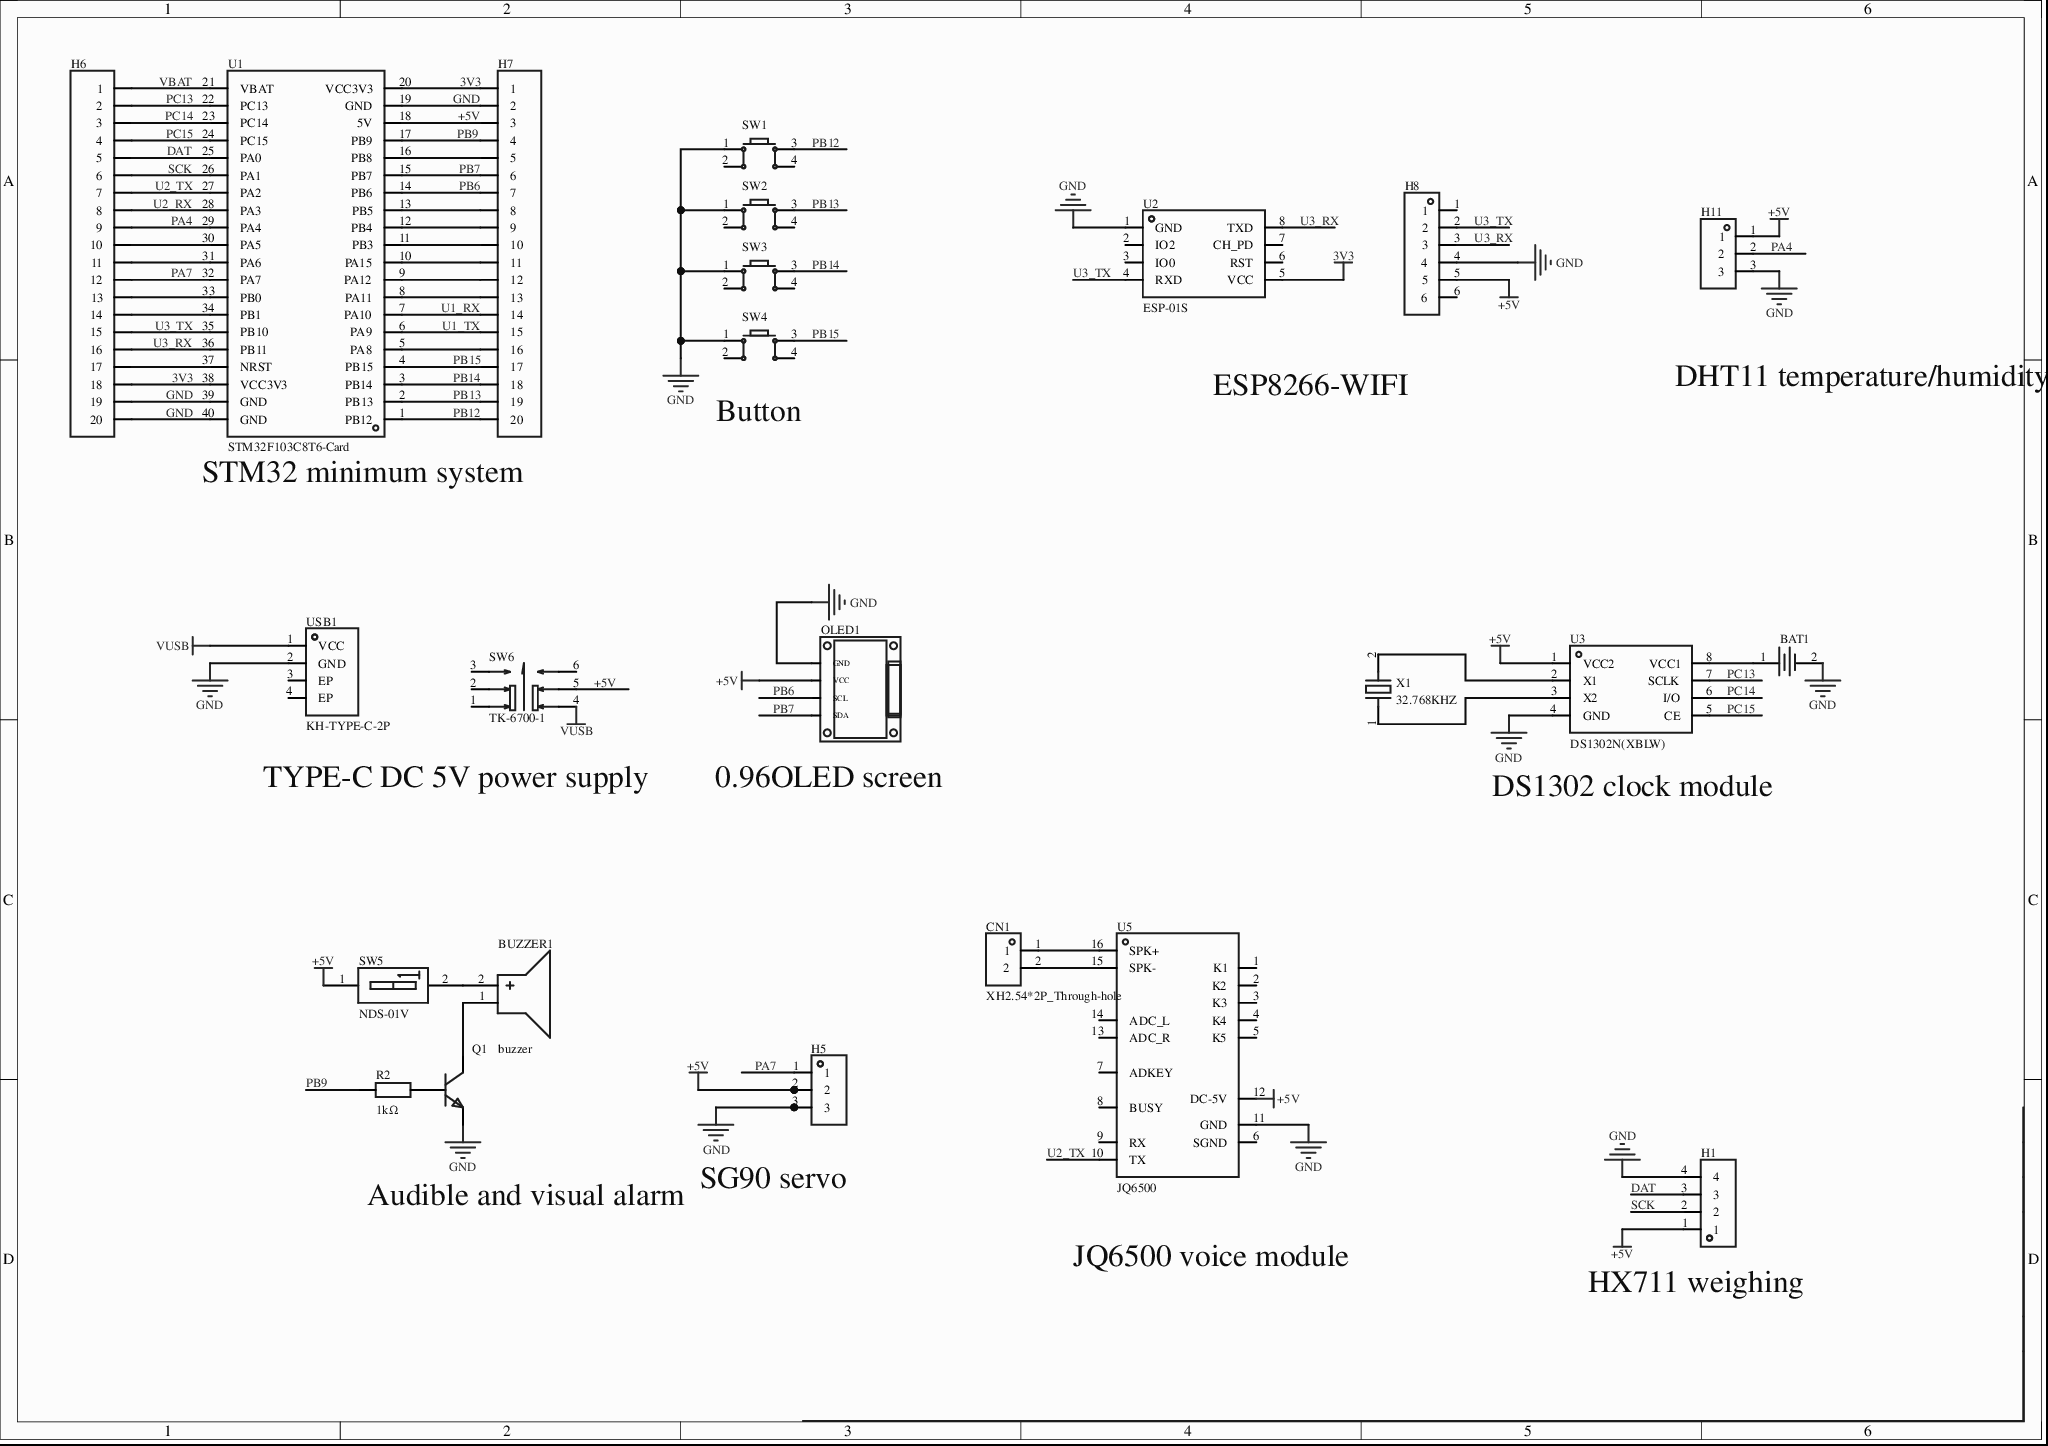
[diagram p0: MISC51988-3.schdoc]
# Altium project MISC51988-2.PrjPcb
1 sheet, 24 parts. Net scope: global (net labels, ports and power ports of the same name join across sheets).
Board file: MISC51988.pcbdoc

## Sheet MISC51988-3.schdoc
size 297 x 209 mm; Version: V1.0; @Project Name: MISC51988; @Page Count: 1; @Update Date: 2026-04-19; @Create Date: 2026-04-19; @Schematic Name: MISC51988; @Page No: 1; @Create Time: 23:22:16; @Update Time: 17:32:40; @Board Name: MISC51988

### Parts
BAT1  KH-BS2032-2-1  [BAT-TH_KH-BS2032-2-1]  (value not drawn)
BUZZER1  buzzer  [BUZ-TH_BD12.0-P6.00-D0.9-RD]
CN1  XH2.54*2P_Through-hole  [CONN-TH_2P-P2.50-XH2.54-2P]
H1  (no value)  [HDR-TH_4P-P2.54-V-F]
H5  (no value)  [HDR-TH_3P-P2.54-V-F]
H6  (no value)  [HDR-TH_20P-P2.54-V-F]
H7  (no value)  [HDR-TH_20P-P2.54-V-F]
H8  (no value)  [HDR-TH_6P-P2.54-V-F]
H11  (no value)  [HDR-TH_3P-P2.54-V-F]
OLED1  (no value)  [0.96OLED_4P]
Q1  (no value)  [S8050_TO_92]
R2  1kΩ  [Res_1/8W]
SW1  (no value)  [SW-TH_4P-L6.0-W6.0-P4.50-LS6.5]
SW2  (no value)  [SW-TH_4P-L6.0-W6.0-P4.50-LS6.5]
SW3  (no value)  [SW-TH_4P-L6.0-W6.0-P4.50-LS6.5]
SW4  (no value)  [SW-TH_4P-L6.0-W6.0-P4.50-LS6.5]
SW5  NDS-01V  [SW-TH_2P-L3.9-W9.9-P2.54-LS7.6]
SW6  TK-6700-1  [SW-TH_TK-6700-1]
U1  STM32F103C8T6-Card  [CONN-TH_L53.3-W22.9_STM32F103C8T6-CARD]
U2  ESP-01S  [WIFIM-TH_ESP-01S]
U3  DS1302N(XBLW)  [PDIP-8_L9.3-W6.4-P2.54-LS7.6-BL]
U5  JQ6500  [MOD-TH_JQ6500]
USB1  KH-TYPE-C-2P  [USB-SMD_KH-TYPE-C-2P]
X1  32.768KHZ  [CRYSTAL-SMD_L3.2-W1.5-1]

### Nets
3V3: H6.18 H7.1 U1.20(VCC3V3) U1.38(VCC3V3) U2.5(VCC)
+5V: H1.1 H5.2 H7.3 H8.5 H11.1 OLED1.2(VCC) SW5.1(A1) SW6.5 U1.18(5V) U3.1(VCC2) U5.12(DC-5V)
GND: BAT1.2 H1.4 H5.3 H6.19 H6.20 H7.2 H8.4 H11.3 OLED1.1(GND) Q1.1(E) SW1.1 SW2.1 SW3.1 SW4.1 U1.19(GND) U1.39(GND) U1.40(GND) U2.1(GND) U3.4(GND) U5.11(GND) USB1.2(GND)
VUSB: SW6.4 USB1.1(VCC)
DAT: H1.3 H6.5 U1.25(PA0)
PA4: H6.9 H11.2 U1.29(PA4)
PA7: H5.1 H6.12 U1.32(PA7)
PB6: H7.7 OLED1.3(SCL) U1.14(PB6)
PB7: H7.6 OLED1.4(SDA) U1.15(PB7)
PB9: H7.4 R2.1 U1.17(PB9)
PB12: H7.20 SW1.3 U1.1(PB12)
PB13: H7.19 SW2.3 U1.2(PB13)
PB14: H7.18 SW3.3 U1.3(PB14)
PB15: H7.17 SW4.3 U1.4(PB15)
PC13: H6.2 U1.22(PC13) U3.7(SCLK)
PC14: H6.3 U1.23(PC14) U3.6(I/O)
PC15: H6.4 U1.24(PC15) U3.5(CE)
SCK: H1.2 H6.6 U1.26(PA1)
U1_RX: H7.14 U1.7(PA10)
U1_TX: H7.15 U1.6(PA9)
U2_RX: H6.8 U1.28(PA3)
U2_TX: H6.7 U1.27(PA2) U5.10(TX)
U3_RX: H6.16 H8.3 U1.36(PB11) U2.8(TXD)
U3_TX: H6.15 H8.2 U1.35(PB10) U2.4(RXD)
VBAT: H6.1 U1.21(VBAT)
NetBAT1_1: BAT1.1 U3.8(VCC1)
NetBUZZER1_1: BUZZER1.1(-) Q1.3(C)
NetBUZZER1_2: BUZZER1.2(+) SW5.2(A2)
NetCN1_1: CN1.1 U5.16(SPK+)
NetCN1_2: CN1.2 U5.15(SPK-)
NetH6_10: H6.10 U1.30(PA5)
NetH6_11: H6.11 U1.31(PA6)
NetH6_13: H6.13 U1.33(PB0)
NetH6_14: H6.14 U1.34(PB1)
NetH6_17: H6.17 U1.37(NRST)
NetH7_5: H7.5 U1.16(PB8)
NetH7_8: H7.8 U1.13(PB5)
NetH7_9: H7.9 U1.12(PB4)
NetH7_10: H7.10 U1.11(PB3)
NetH7_11: H7.11 U1.10(PA15)
NetH7_12: H7.12 U1.9(PA12)
NetH7_13: H7.13 U1.8(PA11)
NetH7_16: H7.16 U1.5(PA8)
NetQ1_2: Q1.2(B) R2.2
NetU3_2: U3.2(X1) X1.2
NetU3_3: U3.3(X2) X1.1

Not connected (* = marked no-connect by the designer): H8 1 6; SW1 2 4; SW2 2 4; SW3 2 4; SW4 2 4; SW6 1* 2* 3* 6*; U2 2(IO2)* 3(IO0)* 6(RST)* 7(CH_PD)*; U5 1(K1) 2(K2) 3(K3) 4(K4) 5(K5) 6(SGND) 7(ADKEY) 8(BUSY) 9(RX) 13(ADC_R) 14(ADC_L); USB1 3(EP) 4(EP)

### Notes on the sheet
- (near SW4) Button
- ESP8266-WIFI
- DHT11 temperature/humidity
- STM32 minimum system
- TYPE-C DC 5V power supply
- (near OLED1) 0.96OLED screen
- (near U3) DS1302 clock module
- Audible and visual alarm
- (near H5) SG90 servo
- JQ6500 voice module
- (near H1) HX711 weighing

### Library data of the parts
BAT1 = KH-BS2032-2-1: Manufacturer: kinghelm(金航标); AddInBom: yes; Symbol: KH-BS2032-2-1; Device: KH-BS2032-2-1; LCSC Part Name: 纽扣电池底座BS-2-1插脚环保; SupplierPart: C3038670; ManufacturerPart: KH-BS2032-2-1; Supplier Footprint: 插件; JLCPCB Part Class: Extended Part; Datasheet: example.com/datasheet/KH-BS2032-2-1/3591728.html; Supplier: LCSC; ConvertToPcb: yes; FootprintName: BAT-TH_KH-BS2032-2-1
BUZZER1 = buzzer: 3D Model: af17e4151ed84fc2a628230bf23763630819f05c4eef4c71ace90d822a990e87; 3D Model Transform: 472.44,472.176,0,270,0,0,0,0,-196.85; AddInBom: yes; Symbol: BUZZER; Device: buzzer; LCSC Part Name: buzzer; Supplier Part: C9900014030; Manufacturer Part: buzzer; Supplier Footprint: buzzer; JLCPCB Part Class: Extended Part; Supplier: LCSC; ConvertToPcb: yes; FootprintName: BUZ-TH_BD12.0-P6.00-D0.9-RD; ModelName: BUZ-TH_BD12.0-P6.00-D0.9-RD
CN1 = XH2.54*2P_直插: 3D Model: 325c595e30db4df8abe76612dd40b0fa0819f05c4eef4c71ace90d822a990e87; 3D Model Transform: 295.275,228.346,0,180,0,0,-0.002,-20.079,-137.795; AddInBom: yes; Symbol: XH2.54*2P_Through-hole; Device: XH2.54*2P_Through-hole; LCSC Part Name: XH2.54*2P_直插; Supplier Part: C9900008615; Manufacturer Part: XH2.54*2P_直插; Supplier Footprint: XH2.54_2P; JLCPCB Part Class: Extended Part; Supplier: LCSC; ConvertToPcb: yes; FootprintName: CONN-TH_2P-P2.50-XH2.54-2P; ModelName: CONN-TH_2P-P2.50-XH2.54-2P
H1 = HDR-F_2.54_1x4P: Symbol: 2.54-1*4P female; ConvertToPcb: yes; ModelId: d187812051054f85879fcaa51a310d8e0819f05c4eef4c71ace90d822a990e87; ModelTransform: 419.6842,98.464,0,0,0,0,0,0,-118.11; Device: HDR-F_2.54_1x4P; AddInBom: yes; SupplierPart: C2718488; Supplier Footprint: 插件; FootprintName: HDR-TH_4P-P2.54-V-F; ModelName: HDR-TH_4P-P2.54-V-F
H5 H11 = HDR-F_2.54_1x3P: Symbol: PM254V-11-03-H85; 3D Model: f3b3cc5aae9641bf9e56fc160cef875b; 3D Model Transform: 299.9994,100,0,0,0,0,0,0,-118.11; ConvertToPcb: yes; ModelName: HDR2.54-F-LI-1X3P; Device: HDR-F_2.54_1x3P; Supplier Part: C541850; Supplier Footprint: 插件; FootprintName: HDR-TH_3P-P2.54-V-F; AddInBom: yes
H6 H7 = HDR-F_2.54_1x20P: ConvertToPcb: yes; ModelId: db7015f7ad9d48b8a3b1188db02e3429; ModelName: HDR-F-2.54_1x20; ModelTransform: 1999.996,100,0,0,0,0,0,0,-118.11; Symbol: HDR-F_2.54_1x20P; Device: HDR-F_2.54_1x20P; AddInBom: yes; SupplierPart: C50984; Supplier Footprint: 插件; FootprintName: HDR-TH_20P-P2.54-V-F
H8 = HDR-F_2.54_1x6P: Symbol: Header-Female-2.54_1x6; ConvertToPcb: yes; ModelId: 0f5bcf94dcda47d085f24cdca1696fe9; ModelTransform: 619.684,94.488,0,0,0,0,0,0,-125.984; Device: HDR-F_2.54_1x6P; AddInBom: yes; SupplierPart: C40877; Supplier Footprint: 插件; FootprintName: HDR-TH_6P-P2.54-V-F; ModelName: HDR-TH_6P-P2.54-V-F
OLED1 = 0.96OLED模块_4P: Device: 0.96OLED module_4P; ConvertToPcb: yes; ModelId: 79c000fdb68d45a296c2e9bedf4f9055; ModelTransform: 1393.69792,1318.895,0,0,0,0,0,-560.079,-137.795; Symbol: 0.96OLED module_4P; FootprintName: 0.96OLED_4P; AddInBom: yes; Supplier Footprint: 插件; ModelName: 0.96OLED_4P
Q1 = S8050_TO_NPN: 3D Model: aafe8e06f2154e7c93506efd0d6632dd; 3D Model Transform: 180.78,141.44,417.3,0,0,0,0,0,-200; ConvertToPcb: yes; ModelName: TO-92-3_L4.9-W3.7-P1.27-L; Symbol: S8050_TO_NPN; Device: S8050_TO_NPN; Supplier Footprint: TO-92; AddInBom: yes; FootprintName: S8050_TO_92
R2 = Res_AXIAL-1/8W: Symbol: Resistor; 3D Model: b2b5ae7ae4c642178fe0039925c86a3f; 3D Model Transform: 282.86,66.88,253.09,0,0,0,0,0,-191; ConvertToPcb: yes; ModelName: RES-TH_BD1.8-L3.2-P7.20-D0.4; Device: Res_AXIAL-1/8W; Supplier Footprint: 轴向引线; Value: 1kΩ; AddInBom: yes; FootprintName: Res_1/8W
SW1-SW4 = Key_TH_6x6x6: Contact current:50mA;Rated voltage(DC):12V;Insulation resistance:100MΩ;Circuit:SPST;Mounting:Through-hole;Button shape:Round;Button/cap colour:Black;Actuating force:260gf@±30gf;Operating temperature:-25℃~+70℃;Pin style:PC pin;Switch length:6mm;Switch width:6mm;Switch height:6mm;With bracket:No;; Symbol: Tact switch; AddInBom: yes; ModelId: 20eee248bc684ccd8cbdbb1d0d91ec6f0819f05c4eef4c71ace90d822a990e87; ModelName: SW-TH_4P-L6.0-W6.0-H5.0-LS6.5-P4.50; ModelTransform: 236.22,323.03,0,90,0,0,0,0,-137.795; Device: Key_TH_6x6x6; FootprintName: SW-TH_4P-L6.0-W6.0-P4.50-LS6.5; ConvertToPcb: yes; Supplier Footprint: 插件
SW5 = NDS-01V_C501305: Forward toggle, high lever; 3D Model: a6fe51954c31461ebc9e88beb6e51f3d0819f05c4eef4c71ace90d822a990e87; 3D Model Transform: 161.417,389.763,0,270,0,0,0,0,-125.984; AddInBom: yes; ModelName: SW-TH_L4.0-W9.9-H5.4-P2.54-B; Symbol: NDS-01V; Device: NDS-01V_C501305; LCSC Part Name: 拨码开关; Supplier Part: C501305; Manufacturer Part: NDS-01V; Supplier Footprint: DIP; JLCPCB Part Class: Extended Part; Supplier: LCSC; ConvertToPcb: yes; FootprintName: SW-TH_2P-L3.9-W9.9-P2.54-LS7.6
SW6 = TK-6700-1: Circuit:DPDT;Self-lock/No-lock:Self-lock;Mounting:Through-hole;Actuating force:2.3N;Operating life:-;; Manufacturer: Yuandi(元迪); AddInBom: yes; ModelId: 1dccfbf2ceb24a728093c1f6ee61932a0819f05c4eef4c71ace90d822a990e87; ModelTransform: 275.59,275.59,0,90,0,0,0,0,-137.795; Circuit: DPDT; Actuator Style: Rectangular plunger; Actuator/Cap Color: Blue; Operating Force: 2.3N; Symbol: TK-6700-1; Device: TK-6700-1; LCSC Part Name: 自锁开关7*7*12.7有声有锁高导高柄插件双排6P按键开关带锁DIP六脚; SupplierPart: C528782; ManufacturerPart: TK-6700-1; Supplier Footprint: 插件; JLCPCB Part Class: Extended Part; Datasheet: example.com/datasheet/TK-6700-1/548571.html; Supplier: LCSC; ConvertToPcb: yes; FootprintName: SW-TH_TK-6700-1; ModelName: SW-TH_TK-6700-1; Self Lock / No Lock: Self-lock; Mounting Type: Through-hole; Termination Style: PC pin; Life: -
U1 = STM32F103C8T6-Card: AddInBom: yes; Device: STM32F103C8T6-Card; Symbol: STM32F103C8T6-CARD; FootprintName: CONN-TH_L53.3-W22.9_STM32F103C8T6-CARD; LCSC Part Name: STM32F103C8T6-Card; SupplierPart: C9900077949; ManufacturerPart: STM32F103C8T6-Card; Supplier Footprint: 插件; Supplier: LCSC; ConvertToPcb: yes
U2 = ESP-01S_C111009: 3D Model: eb7175da78ae48b3b1568cfe3027405f0819f05c4eef4c71ace90d822a990e87; 3D Model Transform: 582.676,976.37608,0,0,0,0,0,388.346,-118.11; AddInBom: yes; Symbol: ESP-01S; Device: ESP-01S_C111009; LCSC Part Name: ESP-01S; Supplier Part: C111009; Manufacturer Part: ESP-01S; Supplier Footprint: -; JLCPCB Part Class: Extended Part; Supplier: LCSC; ConvertToPcb: yes; FootprintName: WIFIM-TH_ESP-01S; ModelName: WIFIM-TH_ESP-01S
U3 = DS1302N(XBLW): Interface type:Three-wire serial interface;Crystal:External;Alarm output:-;; Manufacturer: XBLW(芯伯乐); AddInBom: yes; ModelId: fe5fd42f66544692923c5fbf1ee41ec70819f05c4eef4c71ace90d822a990e87; ModelName: PDIP-8_L10.2-W5.9-H4.5-P2.54-LS7.6-BL; ModelTransform: 364.173,311.8104,0,0,0,0,0,0,-118.11; Voltage - Supply: 2V~5.5V; Current - Supply: 1uA; Symbol: DS1302N(XBLW); Device: DS1302N(XBLW); LCSC Part Name: DS1302N(XBLW); SupplierPart: C42395632; ManufacturerPart: DS1302N(XBLW); Supplier Footprint: DIP-8; JLCPCB Part Class: Extended Part; Datasheet: example.com/upload/public/pdf/source/20241125/ED583BD048AAE751CB9F5E4637775452.pdf; Supplier: LCSC; ConvertToPcb: yes; FootprintName: PDIP-8_L9.3-W6.4-P2.54-LS7.6-BL; Interface: Three-wire serial interface; crystal oscillator: External; Alarm Output: -; Operating Temperature: -40℃~+85℃
U5 = JQ6500: AddInBom: yes; ModelId: c082593c23304ab39aca19a82febcdf20819f05c4eef4c71ace90d822a990e87; ModelTransform: 709.999,864.99827,0,0,0,0,0,0,-196.85; Symbol: JQ6500; Device: JQ6500; LCSC Part Name: JQ6500; SupplierPart: C9900152298; ManufacturerPart: JQ6500; Supplier Footprint: JQ6500-16P; Supplier: LCSC; ConvertToPcb: yes; FootprintName: MOD-TH_JQ6500; ModelName: MOD-TH_JQ6500
USB1 = KH-TYPE-C-2P: Connector type:Type-C;Protocol standard:-;Gender:-;Mounting:Right angle;Contacts:2P;Ports:1;Rated current - power:3A;Operating temperature:-25℃~+85℃;; Manufacturer: kinghelm(金航标); AddInBom: yes; ModelId: 4464b34a7d0f48c2b8c2350e914c93f50819f05c4eef4c71ace90d822a990e87; ModelTransform: 352.362,255.31449,0,0,0,0,0,-49.213,-98.425; Connector Type: Type-C; Number of Contacts: 2P; Number of Ports: 1; Current Rating-Power: 3A; Voltage Rating: 20V; Connect-Disconnect Life: 5 thousand times; Symbol: KH-TYPE-C-2P; Device: KH-TYPE-C-2P; LCSC Part Name: Type-C 弯插; SupplierPart: C2919656; ManufacturerPart: KH-TYPE-C-2P; Supplier Footprint: 插件; JLCPCB Part Class: Extended Part; Datasheet: example.com/datasheet/KH-TYPE-C-2P/3222638.html; Supplier: LCSC; ConvertToPcb: yes; FootprintName: USB-SMD_KH-TYPE-C-2P; ModelName: USB-SMD_KH-TYPE-C-2P; Protocol Standard: -; Gender: -; Mounting Type: Right angle; Length: 6.43mm; Operating Temperature: -25℃~+85℃
X1 = 32.768KHZ: Symbol: 32.768KHZ_C9900023773; AddInBom: yes; ModelId: 762d7afc596f4558a373612390f4386d0819f05c4eef4c71ace90d822a990e87; ModelTransform: 125.984,59.055,0,0,0,0,0,0,0; Device: 32.768KHZ; LCSC Part Name: 32.768KHZ; SupplierPart: C9900023773; ManufacturerPart: 32.768KHZ; Supplier Footprint: FC-135; JLCPCB Part Class: Extended Part; Supplier: LCSC; ConvertToPcb: yes; FootprintName: CRYSTAL-SMD_L3.2-W1.5-1; ModelName: CRYSTAL-SMD_L3.2-W1.5-1